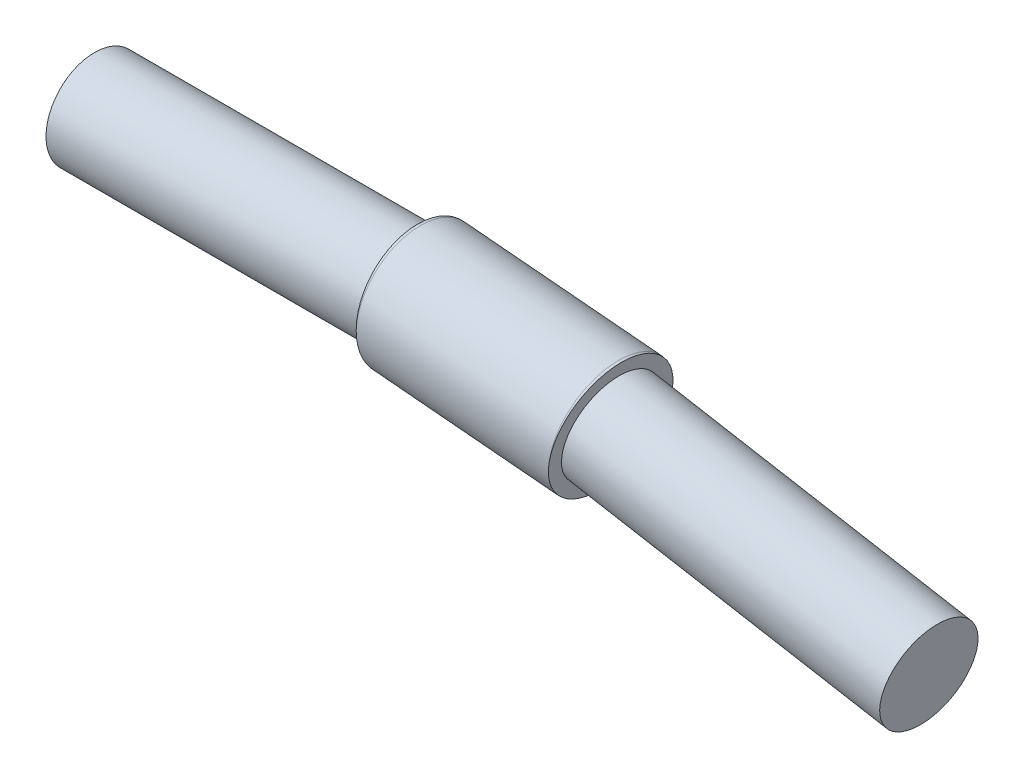
from build123d import *

# Parameters (mm, degrees)
SKETCH_2_R          = 9.5
SKETCH_3_OUTSIDE_W  = 48.11
SKETCH_3_OUTSIDE_H  = 59.263
SKETCH_3_OUTSIDE_R  = 7.5
CUT_EXTRUDE_1_DEPTH = 50
SKETCH_4_OUTSIDE_W  = 48.11
SKETCH_4_OUTSIDE_H  = 81.514
SKETCH_4_OUTSIDE_R  = 7.5
CUT_EXTRUDE_2_DEPTH = 50


with BuildPart() as part:
    # 扫描1: sweep along a path in 草图1
    with BuildLine(Plane.XY) as sweep_1_path:
        Line((0, 0), (50, 0))
        Line((50, 0), (79.885840943, -2.614672282))
        Line((79.885840943, -2.614672282), (129.126228593, -11.297081166))
    # 草图2 → 扫描1 (sweep)
    with BuildSketch(Plane(origin=(0, 0, 0), x_dir=(0, 0, -1), z_dir=(1, 0, 0))):
        Circle(SKETCH_2_R)
    sweep(path=sweep_1_path.line, transition=Transition.RIGHT)

    # 草图3 outside → 切除-拉伸1 (cut)
    with BuildSketch(Plane.ZY):
        with Locations((0, -5.5765)):
            Rectangle(SKETCH_3_OUTSIDE_W, SKETCH_3_OUTSIDE_H)
        Circle(SKETCH_3_OUTSIDE_R, mode=Mode.SUBTRACT)
    extrude(amount=-CUT_EXTRUDE_1_DEPTH, mode=Mode.SUBTRACT)

    # 草图4 outside → 切除-拉伸2 (cut)
    with BuildSketch(Plane(origin=(127.164511036, -22.422534284, 0), x_dir=(0, 0, -1), z_dir=(0.984807753012208, -0.173648177666931, 0))):
        with Locations((0, 5.863)):
            Rectangle(SKETCH_4_OUTSIDE_W, SKETCH_4_OUTSIDE_H)
        with Locations(Location((0, 11.297081166, 0), (0, 0, 90))):
            Circle(SKETCH_4_OUTSIDE_R, mode=Mode.SUBTRACT)
    extrude(amount=-CUT_EXTRUDE_2_DEPTH, mode=Mode.SUBTRACT)


solid = part.part
